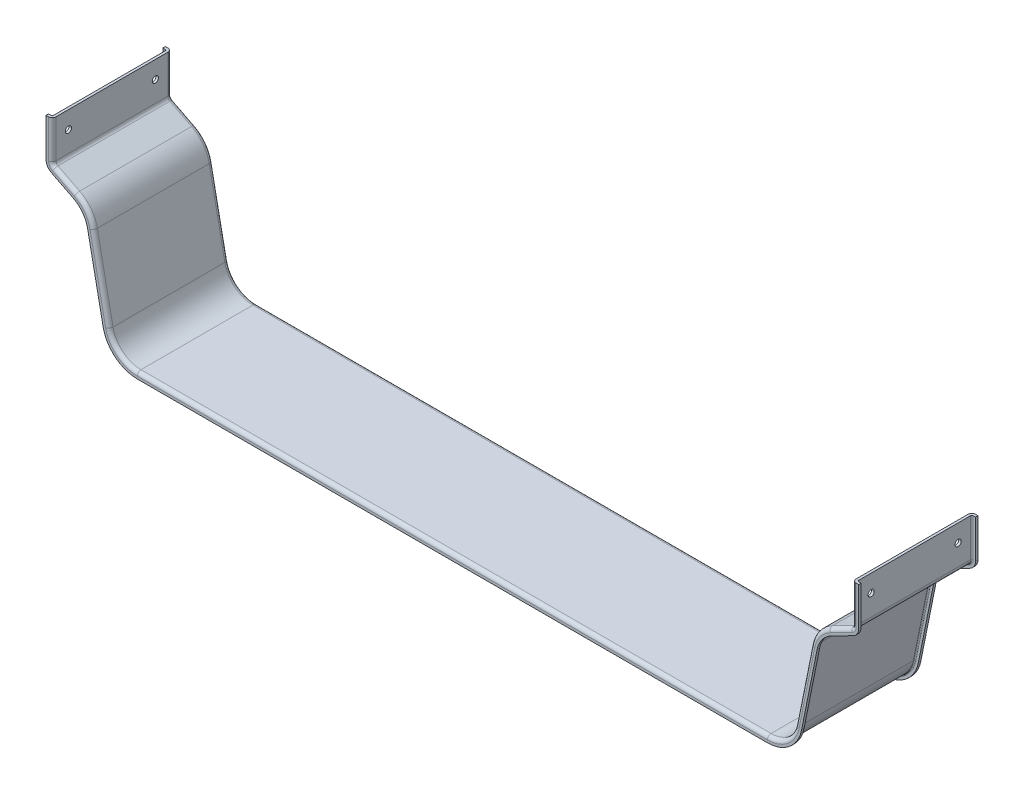
SolidWorks part; units mm, degrees
ref_plane "Front Plane" through (0, 0, 0) normal (0, 0, 1) x (1, 0, 0)
ref_plane "Top Plane" through (0, 0, 0) normal (0, 1, 0) x (1, 0, 0)
ref_plane "Right Plane" through (0, 0, 0) normal (1, 0, 0) x (0, 0, -1)
ref_plane "Plane1" through (0, 0, 96) normal (0, 0, 1) x (1, 0, 0)
sketch "Sketch1" plane through (0, 0, 96) normal (0, 0, 1) x (1, 0, 0)
  line L0 (-1461.4821, 336.2125) -> (-1461.4821, 48.2125)
  line L1 (-1461.4821, 48.2125) -> (-159.4805, 48.2125)
  line L2 (-159.4805, 48.2125) -> (-159.4805, 336.2125)
  line L3 (-159.4805, 336.2125) -> (-1461.4821, 336.2125)
extrude "Boss-Extrude1" add sketch "Sketch1" against normal blind 192
sketch "Sketch2" plane through (0, 336.2125, 0) normal (0, 1, 0) x (-1, 0, 0)
  line L0 (165.4805, -96) -> (165.4805, 92)
  line L1 (165.4805, 92) -> (159.4805, 92)
  line L2 (159.4805, 92) -> (159.4805, -96)
  line L3 (159.4805, -96) -> (165.4805, -96)
extrude "Cut-Extrude1" cut sketch "Sketch2" against normal through all
ref_plane "Plane2" through (0, 0, 92) normal (0, 0, 1) x (1, 0, 0)
sketch "Sketch3" plane through (0, 0, 92) normal (0, 0, 1) x (1, 0, 0)
  line L0 (-165.4805, 48.2125) -> (-165.4805, 268.7125)
  line L1 (-165.4805, 268.7125) -> (-227.4805, 237.2125)
  line L2 (-227.4805, 237.2125) -> (-265.4805, 48.2125)
  line L3 (-265.4805, 48.2125) -> (-165.4805, 48.2125)
extrude "Cut-Extrude2" cut sketch "Sketch3" against normal blind 184
sketch "Sketch4" plane through (0, 48.2125, 0) normal (0, -1, 0) x (1, 0, 0)
  line L0 (-1461.4821, 96) -> (-159.4805, 96)
  line L1 (-159.4805, 96) -> (-159.4805, 92)
  line L2 (-159.4805, 92) -> (-1461.4821, 92)
  line L3 (-1461.4821, 92) -> (-1461.4821, 96)
extrude "Boss-Extrude2" add sketch "Sketch4" along normal blind 6
sketch "Sketch5" plane through (0, 0, 92) normal (0, 0, 1) x (1, 0, 0)
  line L0 (-1461.4821, 268.7125) -> (-1461.4821, 48.2125)
  line L1 (-1461.4821, 48.2125) -> (-1361.4821, 48.2125)
  line L2 (-1361.4821, 48.2125) -> (-1399.4821, 237.2125)
  line L3 (-1399.4821, 237.2125) -> (-1461.4821, 268.7125)
extrude "Cut-Extrude3" cut sketch "Sketch5" against normal blind 184
sketch "Sketch6" plane through (-1461.4821, 0, 0) normal (-1, 0, 0) x (0, 0, 1)
  line L0 (92, 42.2125) -> (92, 336.2125)
  line L1 (92, 336.2125) -> (96, 336.2125)
  line L2 (96, 336.2125) -> (96, 42.2125)
  line L3 (96, 42.2125) -> (92, 42.2125)
extrude "Boss-Extrude3" add sketch "Sketch6" along normal blind 6
sketch "Sketch7" plane through (-165.4805, 0, 0) normal (1, 0, 0) x (0, 0, -1)
  line L0 (92, 48.2125) -> (92, 336.2125)
  line L1 (92, 336.2125) -> (96, 336.2125)
  line L2 (96, 336.2125) -> (96, 48.2125)
  line L3 (96, 48.2125) -> (92, 48.2125)
extrude "Boss-Extrude4" add sketch "Sketch7" along normal blind 6
sketch "Sketch8" plane through (0, 48.2125, 0) normal (0, -1, 0) x (1, 0, 0)
  line L0 (-1461.4821, -92) -> (-159.4805, -92)
  line L1 (-159.4805, -92) -> (-159.4805, -96)
  line L2 (-159.4805, -96) -> (-1461.4821, -96)
  line L3 (-1461.4821, -96) -> (-1461.4821, -92)
extrude "Boss-Extrude5" add sketch "Sketch8" along normal blind 6
sketch "Sketch9" plane through (-1461.4821, 0, 0) normal (-1, 0, 0) x (0, 0, 1)
  line L0 (-96, 42.2125) -> (-96, 336.2125)
  line L1 (-96, 336.2125) -> (-92, 336.2125)
  line L2 (-92, 336.2125) -> (-92, 42.2125)
  line L3 (-92, 42.2125) -> (-96, 42.2125)
extrude "Boss-Extrude6" add sketch "Sketch9" along normal blind 6
sketch "Sketch10" plane through (0, 0, 92) normal (0, 0, -1) x (-1, 0, 0)
  line L0 (222.1712, 233.18) -> (159.4805, 265.031)
  line L1 (159.4805, 265.031) -> (159.4805, 42.2125)
  line L2 (159.4805, 42.2125) -> (260.5668, 42.2125)
  line L3 (260.5668, 42.2125) -> (222.1712, 233.18)
extrude "Cut-Extrude4" cut sketch "Sketch10" against normal through all
sketch "Sketch11" plane through (0, 0, 96) normal (0, 0, 1) x (1, 0, 0)
  line L0 (-1404.7914, 233.18) -> (-1467.4821, 265.031)
  line L1 (-1467.4821, 265.031) -> (-1467.4821, 42.2125)
  line L2 (-1467.4821, 42.2125) -> (-1366.3959, 42.2125)
  line L3 (-1366.3959, 42.2125) -> (-1404.7914, 233.18)
extrude "Cut-Extrude5" cut sketch "Sketch11" against normal up to next
sketch "Sketch12" plane through (0, 0, -96) normal (0, 0, -1) x (-1, 0, 0)
  line L0 (1457.4821, 336.2125) -> (169.4805, 336.2125)
  line L1 (169.4805, 336.2125) -> (169.4805, 271.1669)
  line L2 (169.4805, 271.1669) -> (231.02, 239.9009)
  line L3 (231.02, 239.9009) -> (268.7563, 52.2125)
  line L4 (268.7563, 52.2125) -> (1358.2063, 52.2125)
  line L5 (1358.2063, 52.2125) -> (1395.9426, 239.9009)
  line L6 (1395.9426, 239.9009) -> (1457.4821, 271.1669)
  line L7 (1457.4821, 271.1669) -> (1457.4821, 336.2125)
extrude "Cut-Extrude6" cut sketch "Sketch12" against normal through all
sketch "Sketch13" plane through (0, 0, -96) normal (0, 0, -1) x (-1, 0, 0)
  line L0 (1467.4821, 265.031) -> (1404.7914, 233.18)
  line L1 (1404.7914, 233.18) -> (1366.3959, 42.2125)
  line L2 (1366.3959, 42.2125) -> (1467.4821, 42.2125)
  line L3 (1467.4821, 42.2125) -> (1467.4821, 265.031)
extrude "Cut-Extrude7" cut sketch "Sketch13" against normal through all
sketch "Sketch14" plane through (0, 0, -96) normal (0, 0, -1) x (-1, 0, 0)
  line L0 (222.1712, 233.18) -> (159.4805, 265.031)
  line L1 (159.4805, 265.031) -> (159.4805, 42.2125)
  line L2 (159.4805, 42.2125) -> (260.5668, 42.2125)
  line L3 (260.5668, 42.2125) -> (222.1712, 233.18)
extrude "Cut-Extrude8" cut sketch "Sketch14" against normal through all
hole_wizard "Ø10.0 (10) Diameter Hole1" positions "Sketch16" profile "Sketch15" hole size "Ø10.0" standard "ANSI Metric"
sketch "Sketch16" plane through (-1461.4821, 0, 0) normal (-1, 0, 0) x (0, 0, 1)
  point P0 (-70, 308.2125)
  point P1 (70, 308.2125)
sketch "Sketch15" plane through (-1461.4821, 308.2125, -70) normal (0, 1, 0) x (0, 0, 1)
  line L0 (0, 0) -> (0, 4)
  line L1 (0, 4) -> (5, 4)
  line L2 (5, 4) -> (5, 0)
  line L5 (5, 0) -> (0, 0)
  line L11 (0, -6.35) -> (0, 107.95) construction
  dimension "通孔孔直径" = 10
  dimension "通孔孔深度" = 4
hole_wizard "Ø10.0 (10) Diameter Hole2" positions "Sketch18" profile "Sketch17" hole size "Ø10.0" standard "ANSI Metric"
sketch "Sketch18" plane through (-165.4805, 0, 0) normal (1, 0, 0) x (0, 0, -1)
  point P0 (70, 308.2125)
  point P1 (-70, 308.2125)
sketch "Sketch17" plane through (-165.4805, 308.2125, -70) normal (0, 1, 0) x (0, 0, -1)
  line L0 (0, 0) -> (0, 1302.0016)
  line L1 (0, 1302.0016) -> (5, 1302.0016)
  line L2 (5, 1302.0016) -> (5, 0)
  line L5 (5, 0) -> (0, 0)
  line L11 (0, -6.35) -> (0, 107.95) construction
  dimension "通孔孔直径" = 10
  dimension "通孔孔深度" = 1302.0016
fillet "Fillet1" radius 44 4 edges at (-222.1712, 233.18, 94) (-1404.7914, 233.18, 94) (-1404.7914, 233.18, -94) (-222.1712, 233.18, -94)
fillet "Fillet2" radius 10 2 edges at (-1461.4821, 268.7125, 0) (-165.4805, 268.7125, 0)
fillet "Fillet3" radius 46 2 edges at (-268.7563, 52.2125, 0) (-1358.2063, 52.2125, 0)
fillet "Fillet4" radius 50 4 edges at (-1399.4821, 237.2125, 0) (-265.4805, 48.2125, 0) (-1361.4821, 48.2125, 0) (-227.4805, 237.2125, 0)
fillet "Fillet5" radius 54 2 edges at (-231.02, 239.9009, 0) (-1395.9426, 239.9009, 0)
fillet "Fillet6" radius 2 26 edges at (-165.4805, 305.5305, 92) (-166.9571, 269.6186, 92) (-188.4175, 257.0591, 92) (-188.4175, 257.0591, -92) (-223.0537, 233.8503, 92) (-244.8322, 150.9104, 92) (-244.8322, 150.9104, -92) (-274.7484, 59.5293, 92) (-813.4813, 48.2125, 92) (-1352.2142, 59.5293, 92) (-1382.1304, 150.9104, 92) (-1382.1304, 150.9104, -92) (-1403.909, 233.8503, 92) (-1438.5451, 257.0591, -92) (-1438.5451, 257.0591, 92) (-1460.0055, 269.6186, 92) (-1461.4821, 305.5305, 92) (-1461.4821, 305.5305, -92) (-1460.0055, 269.6186, -92) (-1403.909, 233.8503, -92) (-1352.2142, 59.5293, -92) (-813.4813, 48.2125, -92) (-274.7484, 59.5293, -92) (-223.0537, 233.8503, -92) (-166.9571, 269.6186, -92) (-165.4805, 305.5305, -92)
fillet "Fillet7" radius 6 24 edges at (-1457.4821, 303.6897, -96) (-1438.3744, 261.459, -96) (-169.4805, 303.6897, -96) (-1400.7236, 236.2696, -96) (-169.4805, 271.1669, 0) (-1378.2089, 151.6989, -96) (-188.5882, 261.459, -96) (-1349.6798, 62.624, -96) (-226.239, 236.2696, -96) (-813.4813, 52.2125, -96) (-248.7538, 151.6989, -96) (-277.2828, 62.624, -96) (-169.4805, 303.6897, 96) (-188.5882, 261.459, 96) (-226.239, 236.2696, 96) (-248.7538, 151.6989, 96) (-277.2828, 62.624, 96) (-813.4813, 52.2125, 96) (-1349.6798, 62.624, 96) (-1378.2089, 151.6989, 96) (-1400.7236, 236.2696, 96) (-1438.3744, 261.459, 96) (-1457.4821, 303.6897, 96) (-1457.4821, 271.1669, 0)
fillet "Fillet8" radius 16 4 edges at (-1467.4821, 265.031, 94) (-1467.4821, 265.031, -94) (-159.4805, 265.031, 94) (-159.4805, 265.031, -94)
fillet "Fillet9" radius 56 4 edges at (-1366.3959, 42.2125, 94) (-1366.3959, 42.2125, -94) (-260.5668, 42.2125, 94) (-260.5668, 42.2125, -94)
